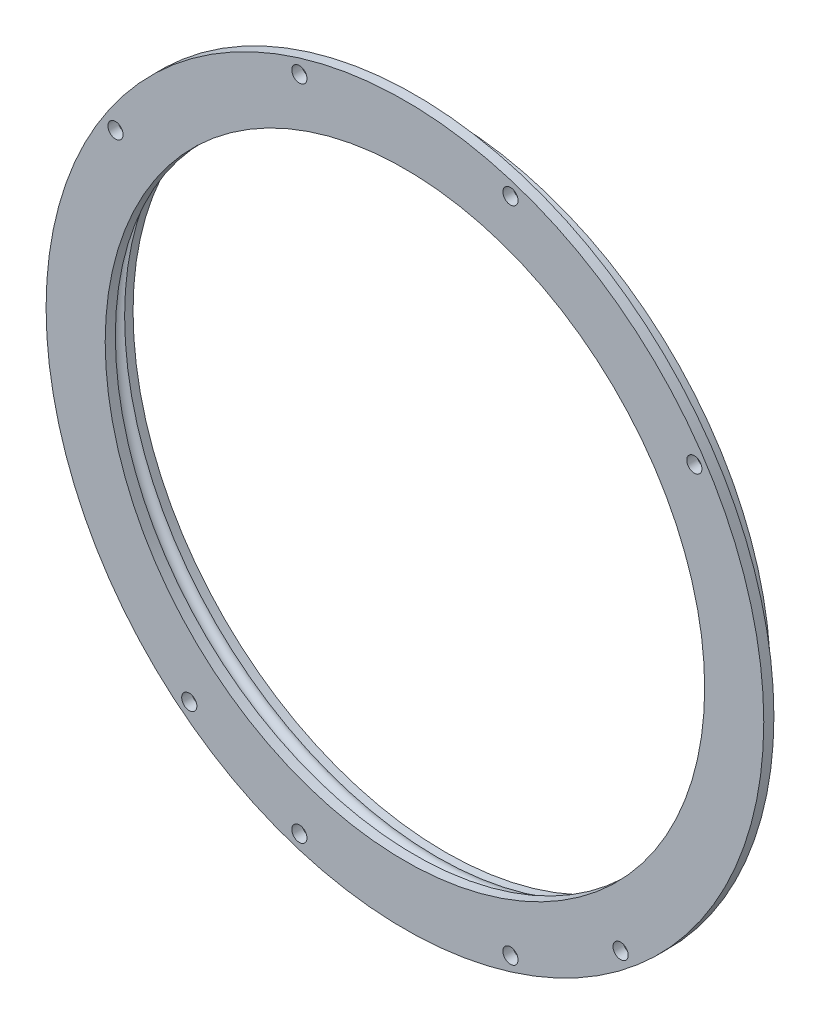
from build123d import *

# Parameters (mm, degrees)
SKETCH_1_R          = 425
SKETCH_1_R_2        = 355
EXTRUDE_2_DEPTH     = 12
SKETCH_3_R          = 385
SKETCH_3_R_2        = 370
EXTRUDE_3_DEPTH     = 36
SWEEP_2_PROFILE_R   = 8
SKETCH_23_W         = 4.5
SKETCH_23_H         = 385
SKETCH_24_R         = 9
CUT_EXTRUDE_1_DEPTH = 15


with BuildPart() as part:
    # 草图1 → 凸台-拉伸2 (new body)
    with BuildSketch(Plane.XY):
        Circle(SKETCH_1_R)
        Circle(SKETCH_1_R_2, mode=Mode.SUBTRACT)
    extrude(amount=EXTRUDE_2_DEPTH)

    # 草图3 → 凸台-拉伸3 (add)
    with BuildSketch(Plane(origin=(0, 0, 0), x_dir=(-1, 0, 0), z_dir=(0, 0, -1))):
        with Locations(Location((0, 0, 0), (0, 0, 180))):
            Circle(SKETCH_3_R)
        Circle(SKETCH_3_R_2, mode=Mode.SUBTRACT)
    extrude(amount=EXTRUDE_3_DEPTH)

    # 切除-扫描2: sweep along a path in 草图4
    with BuildLine(Plane.XY.offset(-18)) as sweep_2_path:
        CenterArc((0, 0), 370, 0, 360)
    # 切除-扫描2 profile (on start of the path) → 切除-扫描2 (sweep, cut)
    with BuildSketch(Plane(origin=(370, 0, -18), x_dir=(0, 0, 1), z_dir=(0, 1, 0))):
        Circle(SWEEP_2_PROFILE_R)
    sweep(path=sweep_2_path.line, mode=Mode.SUBTRACT)

    # 草图23 → M10x1.0 螺纹孔1 (revolve, cut)
    with BuildSketch(Plane(origin=(0, 0, -18), x_dir=(0, 0, 1), z_dir=(0, 1, 0))):
        with Locations((2.25, 192.5)):
            Rectangle(SKETCH_23_W, SKETCH_23_H)
    revolve(axis=Axis((-6.35, 0, -18), (1, 0, 0)), mode=Mode.SUBTRACT)

    # 草图24 → 切除-拉伸1 (cut)
    with BuildSketch(Plane(origin=(0, 0, 0), x_dir=(-1, 0, 0), z_dir=(0, 0, -1))):
        with Locations((-125, -389.430353208)):
            Circle(SKETCH_24_R)
        with Locations((125, -389.430353208)):
            Circle(SKETCH_24_R)
        with Locations((-255.40902876, -319.448318243)):
            Circle(SKETCH_24_R)
        with Locations((255.40902876, -319.448318243)):
            Circle(SKETCH_24_R)
        with Locations((-125, 389.430353208)):
            Circle(SKETCH_24_R)
        with Locations((125, 389.430353208)):
            Circle(SKETCH_24_R)
        with Locations((342.768366919, 223.138626507)):
            Circle(SKETCH_24_R)
        with Locations((-342.768366919, 223.138626507)):
            Circle(SKETCH_24_R)
    extrude(amount=-CUT_EXTRUDE_1_DEPTH, mode=Mode.SUBTRACT)


solid = part.part
